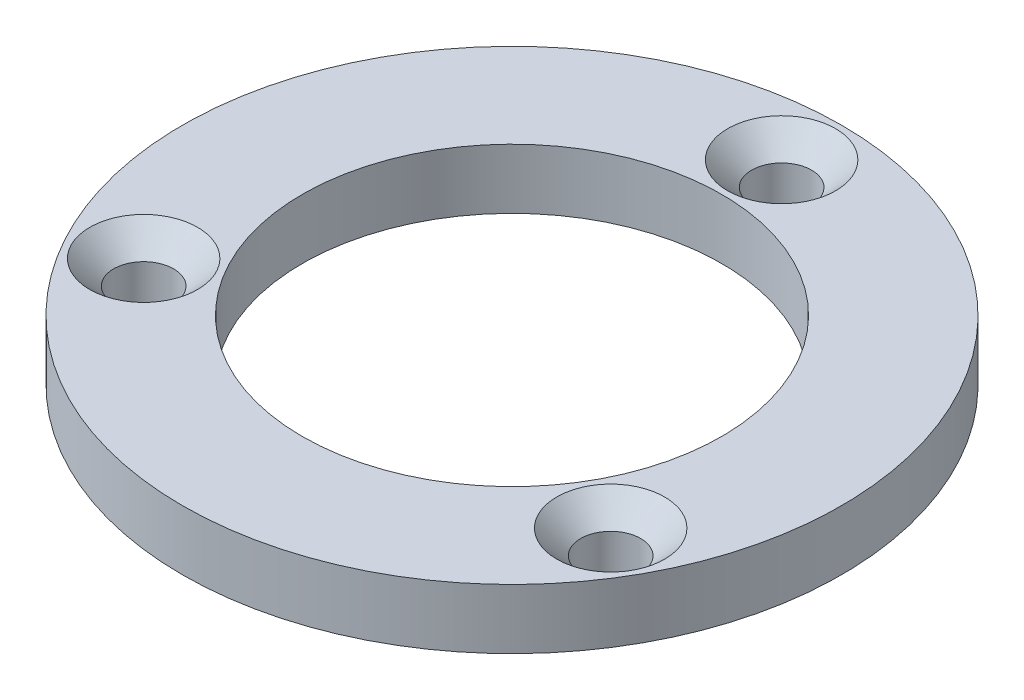
SolidWorks part; units mm, degrees
ref_plane "Front Plane" through (0, 0, 0) normal (0, 0, 1) x (1, 0, 0)
ref_plane "Top Plane" through (0, 0, 0) normal (0, 1, 0) x (1, 0, 0)
ref_plane "Right Plane" through (0, 0, 0) normal (1, 0, 0) x (0, 0, -1)
other "Configuration Table"
sketch "Sketch1" plane through (0, 0, 0) normal (0, 1, 0) x (1, 0, 0)
  circle A0 centre (0, 0) radius 27.5
  circle A1 centre (0, 0) radius 17.5
  dimension "D1" = 55
  dimension "D2" = 35
extrude "Boss-Extrude1" add sketch "Sketch1" along normal blind 5
sketch "Sketch2" plane through (0, 5, 0) normal (0, 1, 0) x (1, 0, 0)
  circle A0 centre (0, 0) radius 22.5
  point P4 (0, 22.5)
  point P10 (19.4856, -11.25)
  point P11 (-19.4856, -11.25)
  dimension "D1" = 45
  dimension "D2" = 3
hole_wizard "Hole1" positions "Sketch2" profile "Sketch3" legacy end condition through all
sketch "Sketch3" plane through (-19.4856, 5, 11.25) normal (1, 0, 0) x (0, 0, 1)
  line L0 (0, 0) -> (0, 5)
  line L1 (0, 5) -> (2.5, 5)
  line L2 (2.5, 5) -> (2.5, 2)
  line L3 (2.5, 2) -> (4.5, 0)
  line L4 (4.5, 0) -> (0, 0)
  line L5 (0, -6.4453) -> (0, 115.525) construction
  line L6 (-2.5, 2) -> (-4.5, 0) construction
  dimension "直径" = 5
  dimension "深度" = 5
  dimension "锥坑角度" = 90
  dimension "锥坑直径" = 9
